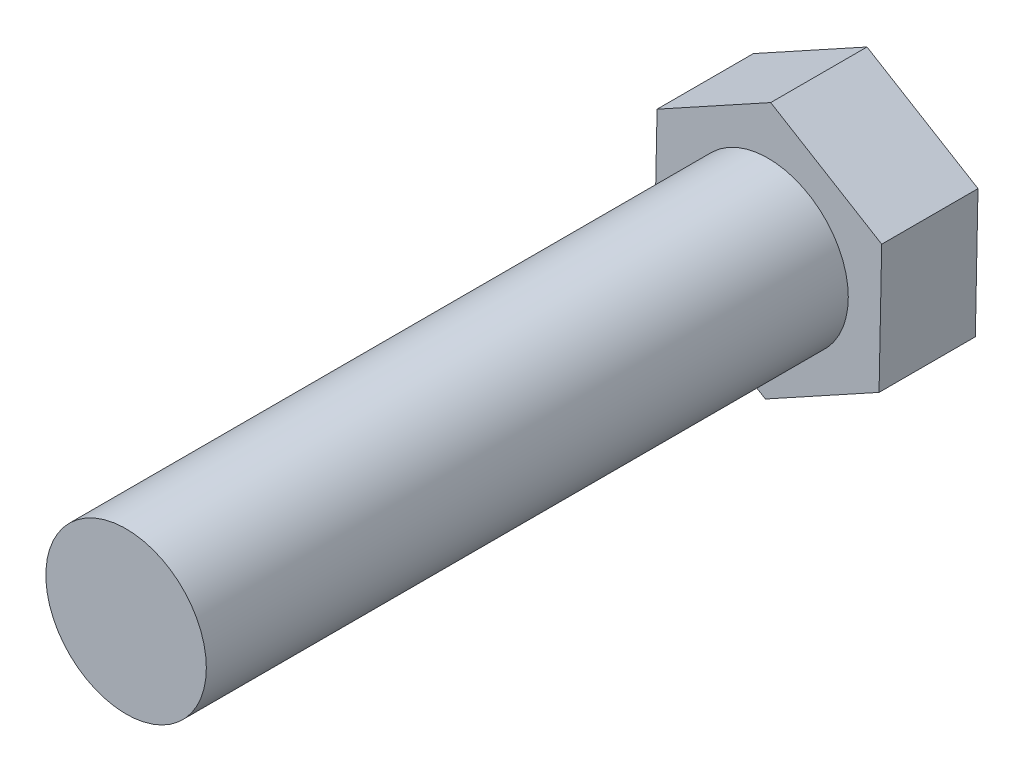
SolidWorks part; units mm, degrees
ref_plane "前视基准面" through (0, 0, 0) normal (0, 0, 1) x (1, 0, 0)
ref_plane "上视基准面" through (0, 0, 0) normal (0, 1, 0) x (1, 0, 0)
ref_plane "右视基准面" through (0, 0, 0) normal (1, 0, 0) x (0, 0, -1)
sketch "草图1" plane through (0, 0, 0) normal (0, 0, 1) x (1, 0, 0)
  circle A0 centre (0, 0) radius 2.5
  dimension "D1" = 5
extrude "凸台-拉伸1" add sketch "草图1" along normal blind 20
sketch "草图2" plane through (0, 0, 0) normal (0, 0, -1) x (-1, 0, 0)
  line L1 (0.0829, -4.0406) -> (3.5407, -1.9485)
  line L2 (3.5407, -1.9485) -> (3.4578, 2.0921)
  line L3 (3.4578, 2.0921) -> (-0.0829, 4.0406)
  line L4 (-0.0829, 4.0406) -> (-3.5407, 1.9485)
  line L5 (-3.5407, 1.9485) -> (-3.4578, -2.0921)
  line L6 (-3.4578, -2.0921) -> (0.0829, -4.0406)
  circle A0 centre (0, 0) radius 3.5 construction
  dimension "D1" = 7
extrude "凸台-拉伸2" add sketch "草图2" along normal blind 3
